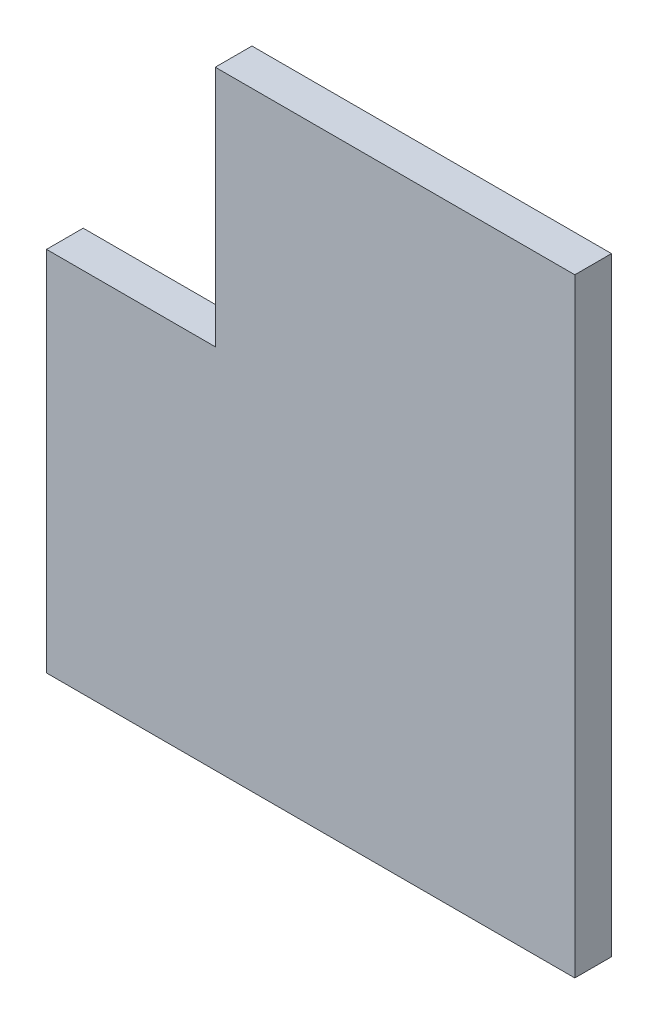
SolidWorks part; units mm, degrees
ref_plane "Front Plane" through (0, 0, 0) normal (0, 0, 1) x (1, 0, 0)
ref_plane "Top Plane" through (0, 0, 0) normal (0, 1, 0) x (1, 0, 0)
ref_plane "Right Plane" through (0, 0, 0) normal (1, 0, 0) x (0, 0, -1)
sketch "Sketch1" plane through (0, 0, 0) normal (0, 0, 1) x (1, 0, 0)
  line L0 (0, 0) -> (0, -415)
  line L1 (0, 0) -> (-245, 0)
  line L4 (-245, 0) -> (-245, -165)
  line L5 (-245, -165) -> (-360, -165)
  line L7 (0, -415) -> (-360, -415)
  line L8 (-360, -165) -> (-360, -415)
  dimension "D1" = 245
  dimension "D2" = 250
  dimension "D3" = 415
  dimension "D4" = 115
extrude "Boss-Extrude1" add sketch "Sketch1" along normal blind 25
